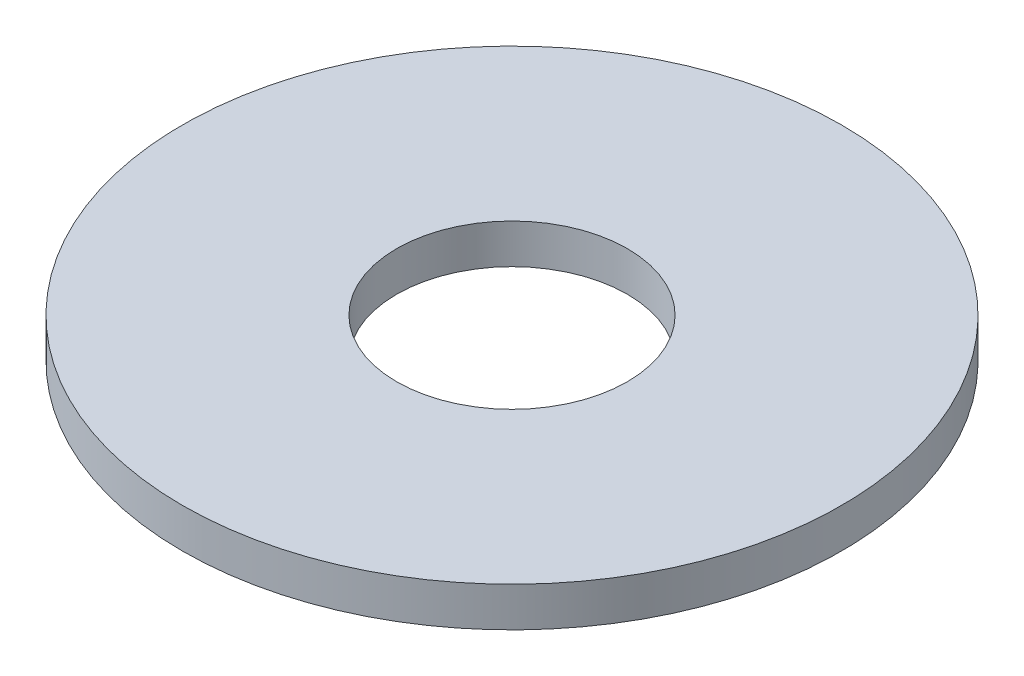
SolidWorks part; units mm, degrees
ref_plane "Front Plane" through (0, 0, 0) normal (0, 0, 1) x (1, 0, 0)
ref_plane "Top Plane" through (0, 0, 0) normal (0, 1, 0) x (1, 0, 0)
ref_plane "Right Plane" through (0, 0, 0) normal (1, 0, 0) x (0, 0, -1)
sketch "Sketch1" plane through (0, 0, 0) normal (0, 1, 0) x (1, 0, 0)
  circle A0 centre (0, 0) radius 25
  circle A1 centre (0, 0) radius 8.75
  dimension "D1" = 17.5
  dimension "D2" = 50
extrude "Boss-Extrude1" add sketch "Sketch1" along normal blind 3
